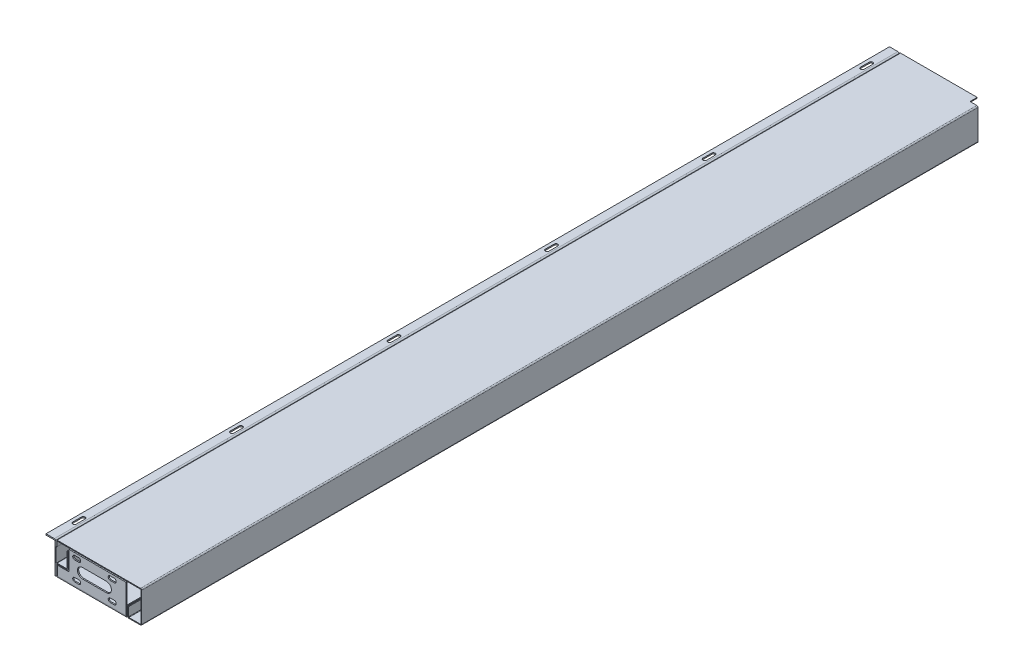
from build123d import *

# Parameters (mm, degrees)
EXTRUDE_1_DEPTH             = 1058
EXTRUDE_2_DEPTH             = 1058
EXTRUDE_2_2_DEPTH           = 1058
EXTRUDE_3_DEPTH             = 3
FILLET_1_R                  = 4
FILLET_2_R                  = 1
FILLET_3_R                  = 1
FILLET_4_R                  = 1
FILLET_5_R                  = 3
FILLET_6_R                  = 3
CUT_EXTRUDE_1_DEPTH         = 2129.398693854
CUT_EXTRUDE_3493_DEPTH      = 3
CUT_EXTRUDE_3714_DEPTH      = 1083.584407795
CUT_EXTRUDE_3714_DEPTH_BACK = 1083.584407795
SKETCH_6_W                  = 20
SKETCH_6_H                  = 18


with BuildPart() as part:
    # 草图1 → 凸台-拉伸1 (new, symmetric)
    with BuildSketch(Plane.XY):
        Polygon((-25, 0), (0, 0), (0, -80), (-3, -80), (-3, -3), (-25, -3), align=None)
    extrude(amount=EXTRUDE_1_DEPTH, both=True)

    # 圆角1
    fillet_1_edges = [part.edges().sort_by_distance(p)[0] for p in [
        (0, 0, 0),
    ]]
    fillet(fillet_1_edges, radius=FILLET_1_R)

    # 圆角2
    fillet_2_edges = [part.edges().sort_by_distance(p)[0] for p in [
        (-3, -3, 0),
    ]]
    fillet(fillet_2_edges, radius=FILLET_2_R)

    # 草图7 → Cut-Extrude 3493 (cut)
    with BuildSketch(Plane(origin=(0, 0, 0), x_dir=(1, 0, 0), z_dir=(0, 1, 0))):
        with BuildLine():
            Line((-17, 977), (-17, 999))
            ThreePointArc((-17, 999), (-12.5, 1003.5), (-8, 999))
            Line((-8, 999), (-8, 977))
            ThreePointArc((-8, 977), (-12.5, 972.5), (-17, 977))
        make_face()
        with BuildLine():
            Line((-17, 581.8), (-17, 603.8))
            ThreePointArc((-17, 603.8), (-12.5, 608.3), (-8, 603.8))
            Line((-8, 603.8), (-8, 581.8))
            ThreePointArc((-8, 581.8), (-12.5, 577.3), (-17, 581.8))
        make_face()
        with BuildLine():
            Line((-17, 186.6), (-17, 208.6))
            ThreePointArc((-17, 208.6), (-12.5, 213.1), (-8, 208.6))
            Line((-8, 208.6), (-8, 186.6))
            ThreePointArc((-8, 186.6), (-12.5, 182.1), (-17, 186.6))
        make_face()
        with BuildLine():
            Line((-17, -208.6), (-17, -186.6))
            ThreePointArc((-17, -186.6), (-12.5, -182.1), (-8, -186.6))
            Line((-8, -186.6), (-8, -208.6))
            ThreePointArc((-8, -208.6), (-12.5, -213.1), (-17, -208.6))
        make_face()
        with BuildLine():
            Line((-17, -603.8), (-17, -581.8))
            ThreePointArc((-17, -581.8), (-12.5, -577.3), (-8, -581.8))
            Line((-8, -581.8), (-8, -603.8))
            ThreePointArc((-8, -603.8), (-12.5, -608.3), (-17, -603.8))
        make_face()
        with BuildLine():
            Line((-17, -999), (-17, -977))
            ThreePointArc((-17, -977), (-12.5, -972.5), (-8, -977))
            Line((-8, -977), (-8, -999))
            ThreePointArc((-8, -999), (-12.5, -1003.5), (-17, -999))
        make_face()
    extrude(amount=-CUT_EXTRUDE_3493_DEPTH, mode=Mode.SUBTRACT)


with BuildPart() as body_2:
    # 草图2 → 凸台-拉伸2 (new, symmetric)
    with BuildSketch(Plane.XY):
        Polygon((0, 0), (0, -15), (2, -15), (2, -2), (213, -2), (213, -78), (182, -78), (182, -55), (180, -55), (180, -80), (215, -80), (215, 0), align=None)
    extrude(amount=EXTRUDE_2_DEPTH, both=True)

    # 圆角3
    fillet_3_edges = [body_2.edges().sort_by_distance(p)[0] for p in [
        (182, -78, 0),
        (213, -78, 0),
        (213, -2, 0),
        (2, -2, 0),
    ]]
    fillet(fillet_3_edges, radius=FILLET_3_R)

    # 圆角5
    fillet_5_edges = [body_2.edges().sort_by_distance(p)[0] for p in [
        (215, 0, 0),
        (215, -80, 0),
        (180, -80, 0),
        (0, 0, 0),
    ]]
    fillet(fillet_5_edges, radius=FILLET_5_R)

    # 草图6 → Cut-Extrude 3714 (cut, two sides: drawn at the far end of the back side and taken through both)
    with BuildSketch(Plane(origin=(0, 0, 0), x_dir=(1, 0, 0), z_dir=(0, 1, 0)).offset(-CUT_EXTRUDE_3714_DEPTH_BACK)):
        with Locations((205, 1049)):
            Rectangle(SKETCH_6_W, SKETCH_6_H)
    extrude(amount=CUT_EXTRUDE_3714_DEPTH + CUT_EXTRUDE_3714_DEPTH_BACK, mode=Mode.SUBTRACT)


with BuildPart() as body_3:
    # 草图2 → Extrude 2 2 (new, symmetric)
    with BuildSketch(Plane.XY):
        Polygon((0, -50), (0, -80), (178.5, -80), (178.5, -55), (176.5, -55), (176.5, -78), (2, -78), (2, -52), (30, -52), (30, -11), (28, -11), (28, -50), align=None)
    extrude(amount=EXTRUDE_2_2_DEPTH, both=True)

    # 圆角4
    fillet_4_edges = [body_3.edges().sort_by_distance(p)[0] for p in [
        (28, -50, 0),
        (2, -52, 0),
        (2, -78, 0),
        (176.5, -78, 0),
    ]]
    fillet(fillet_4_edges, radius=FILLET_4_R)

    # 圆角6
    fillet_6_edges = [body_3.edges().sort_by_distance(p)[0] for p in [
        (30, -52, 0),
        (178.5, -80, 0),
        (0, -80, 0),
        (0, -50, 0),
    ]]
    fillet(fillet_6_edges, radius=FILLET_6_R)


with BuildPart() as body_4:
    # 草图3 → 凸台-拉伸3 (new body)
    with BuildSketch(Plane.XY.offset(1058)):
        Polygon((175.5, -78), (175.5, -5), (33, -5), (33, -54), (4, -54), (4, -78), align=None)
    extrude(amount=-EXTRUDE_3_DEPTH)

    # 草图5 → 切除-拉伸1 (cut, through all)
    with BuildSketch(Plane.XY.offset(1058)):
        with BuildLine():
            Line((47, -11), (57, -11))
            ThreePointArc((57, -11), (62, -16), (57, -21))
            Line((57, -21), (47, -21))
            ThreePointArc((47, -21), (42, -16), (47, -11))
        make_face()
        with BuildLine():
            Line((47, -69), (57, -69))
            ThreePointArc((57, -69), (62, -64), (57, -59))
            Line((57, -59), (47, -59))
            ThreePointArc((47, -59), (42, -64), (47, -69))
        make_face()
        with BuildLine():
            Line((136, -11), (146, -11))
            ThreePointArc((146, -11), (151, -16), (146, -21))
            Line((146, -21), (136, -21))
            ThreePointArc((136, -21), (131, -16), (136, -11))
        make_face()
        with BuildLine():
            Line((136, -69), (146, -69))
            ThreePointArc((146, -69), (151, -64), (146, -59))
            Line((146, -59), (136, -59))
            ThreePointArc((136, -59), (131, -64), (136, -69))
        make_face()
        with BuildLine():
            Line((126.5, -52.5), (66.5, -52.5))
            ThreePointArc((66.5, -52.5), (54, -40), (66.5, -27.5))
            Line((66.5, -27.5), (126.5, -27.5))
            ThreePointArc((126.5, -27.5), (139, -40), (126.5, -52.5))
        make_face()
    extrude(amount=-CUT_EXTRUDE_1_DEPTH, mode=Mode.SUBTRACT)


with BuildPart() as body_5:
    # 镜向1: mirrored copy
    add(body_4.part.mirror(Plane.XY))


solid = Compound([part.part, body_2.part, body_3.part, body_4.part, body_5.part])
